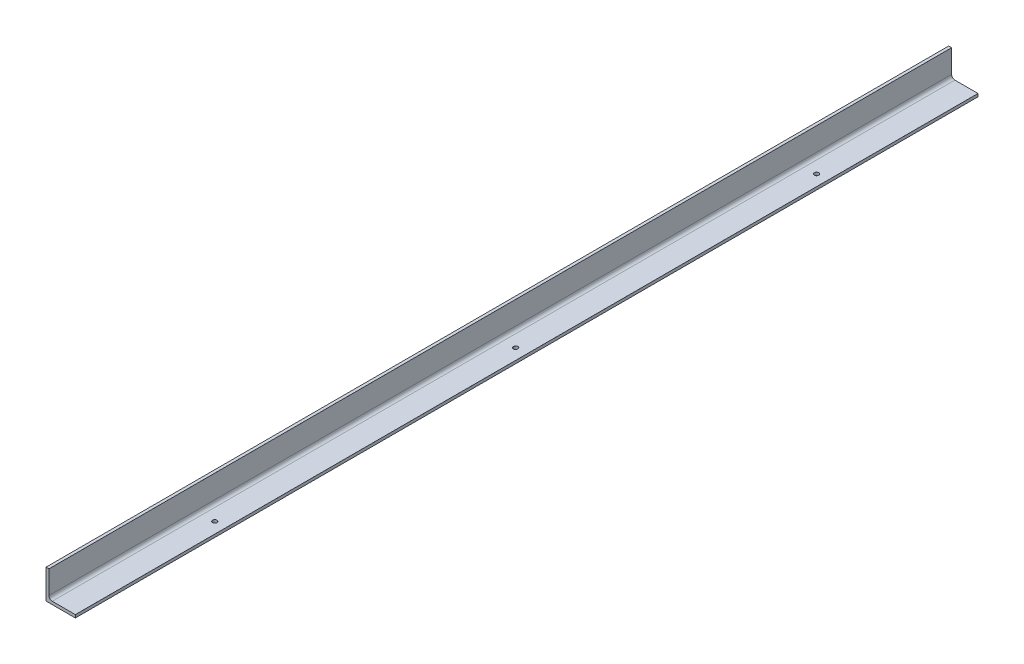
SolidWorks part; units mm, degrees
material "热轧等边角钢 Q235A"
ref_plane "前视基准面" through (0, 0, 0) normal (0, 0, 1) x (1, 0, 0)
ref_plane "上视基准面" through (0, 0, 0) normal (0, 1, 0) x (1, 0, 0)
ref_plane "右视基准面" through (0, 0, 0) normal (1, 0, 0) x (0, 0, -1)
sketch "草图1" plane through (0, 0, 0) normal (0, 0, 1) x (1, 0, 0)
  line L0 (0, 0) -> (0, 40)
  line L1 (0, 40) -> (3.99, 40)
  line L2 (4, 39.99) -> (4, 8.5)
  line L3 (8.5, 4) -> (39.99, 4)
  line L4 (40, 3.99) -> (40, 0)
  line L5 (40, 0) -> (0, 0)
  arc A0 (4, 39.99) -> (3.99, 40) centre (3.99, 39.99) ccw
  arc A1 (8.5, 4) -> (4, 8.5) centre (8.5, 8.5) cw
  arc A2 (40, 3.99) -> (39.99, 4) centre (39.99, 3.99) ccw
  point P9 (4, 40)
  point P14 (40, 4)
extrude "拉伸1" add sketch "草图1" along normal blind 1230
ref_plane "基准面1" through (0, 0, 1126) normal (0, 0, 1) x (1, 0, 0)
hole_wizard "Ø6.0 (6) 直径孔1" positions "草图11" profile "草图10" hole size "Ø6.0" standard "Gb" end condition through all
sketch "草图11" plane through (0, 0, 0) normal (0, -1, 0) x (-1, 0, 0)
  line L0 (-40, -1230) -> (-40, 0) construction
  line L1 (0, 0) -> (-40, 0) construction
  point P0 (-25, -205)
  dimension "D1" = 15
  dimension "D2" = 205
sketch "草图10" plane through (25, 0, 205) normal (1, 0, 0) x (0, 0, -1)
  line L0 (0, 0) -> (0, 40)
  line L1 (0, 40) -> (3, 40)
  line L2 (3, 40) -> (3, 0)
  line L5 (3, 0) -> (0, 0)
  line L11 (0, -6.35) -> (0, 107.95) construction
  dimension "通孔孔直径" = 6
  dimension "通孔孔深度" = 40
pattern_linear "阵列(线性)1" count 3 spacing 410 along (0, 0, 1) of "Ø6.0 (6) 直径孔1"
equation "\"D2@草图1\" = \"D1@草图1\""
equation "\"D4@草图1\" = \"D3@草图1\""
equation "\"D7@草图1\" = \"D5@草图1\""
